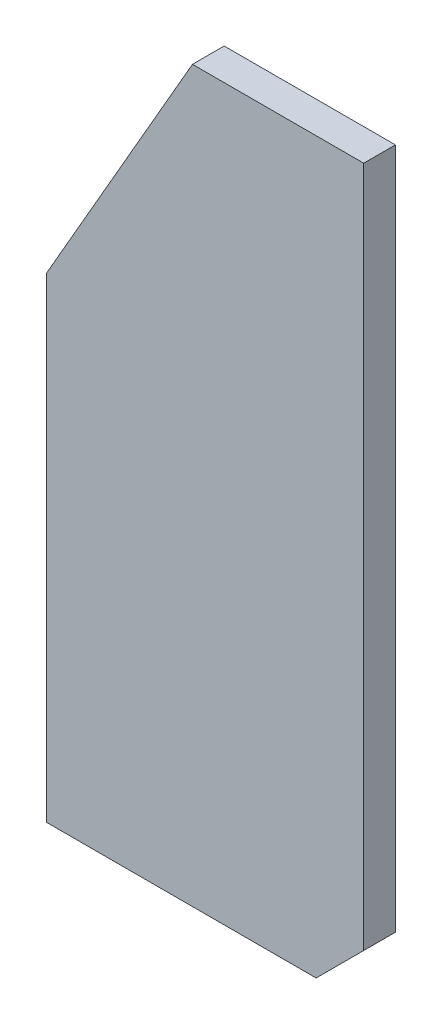
from build123d import *

# Parameters (mm, degrees)
EXTRUDE_1_DEPTH = 5
CHAMFER_1_SIZE  = 15


with BuildPart() as part:
    # 草图1 → 凸台-拉伸1 (new, symmetric)
    with BuildSketch(Plane.XY):
        Polygon((0, 0), (0, 150), (46, 230), (100, 230), (100, 0), align=None)
    extrude(amount=EXTRUDE_1_DEPTH, both=True)

    # 倒角1
    chamfer_1_edges = [part.edges().sort_by_distance(p)[0] for p in [
        (100, 0, 0),
    ]]
    chamfer(chamfer_1_edges, length=CHAMFER_1_SIZE)


solid = part.part
